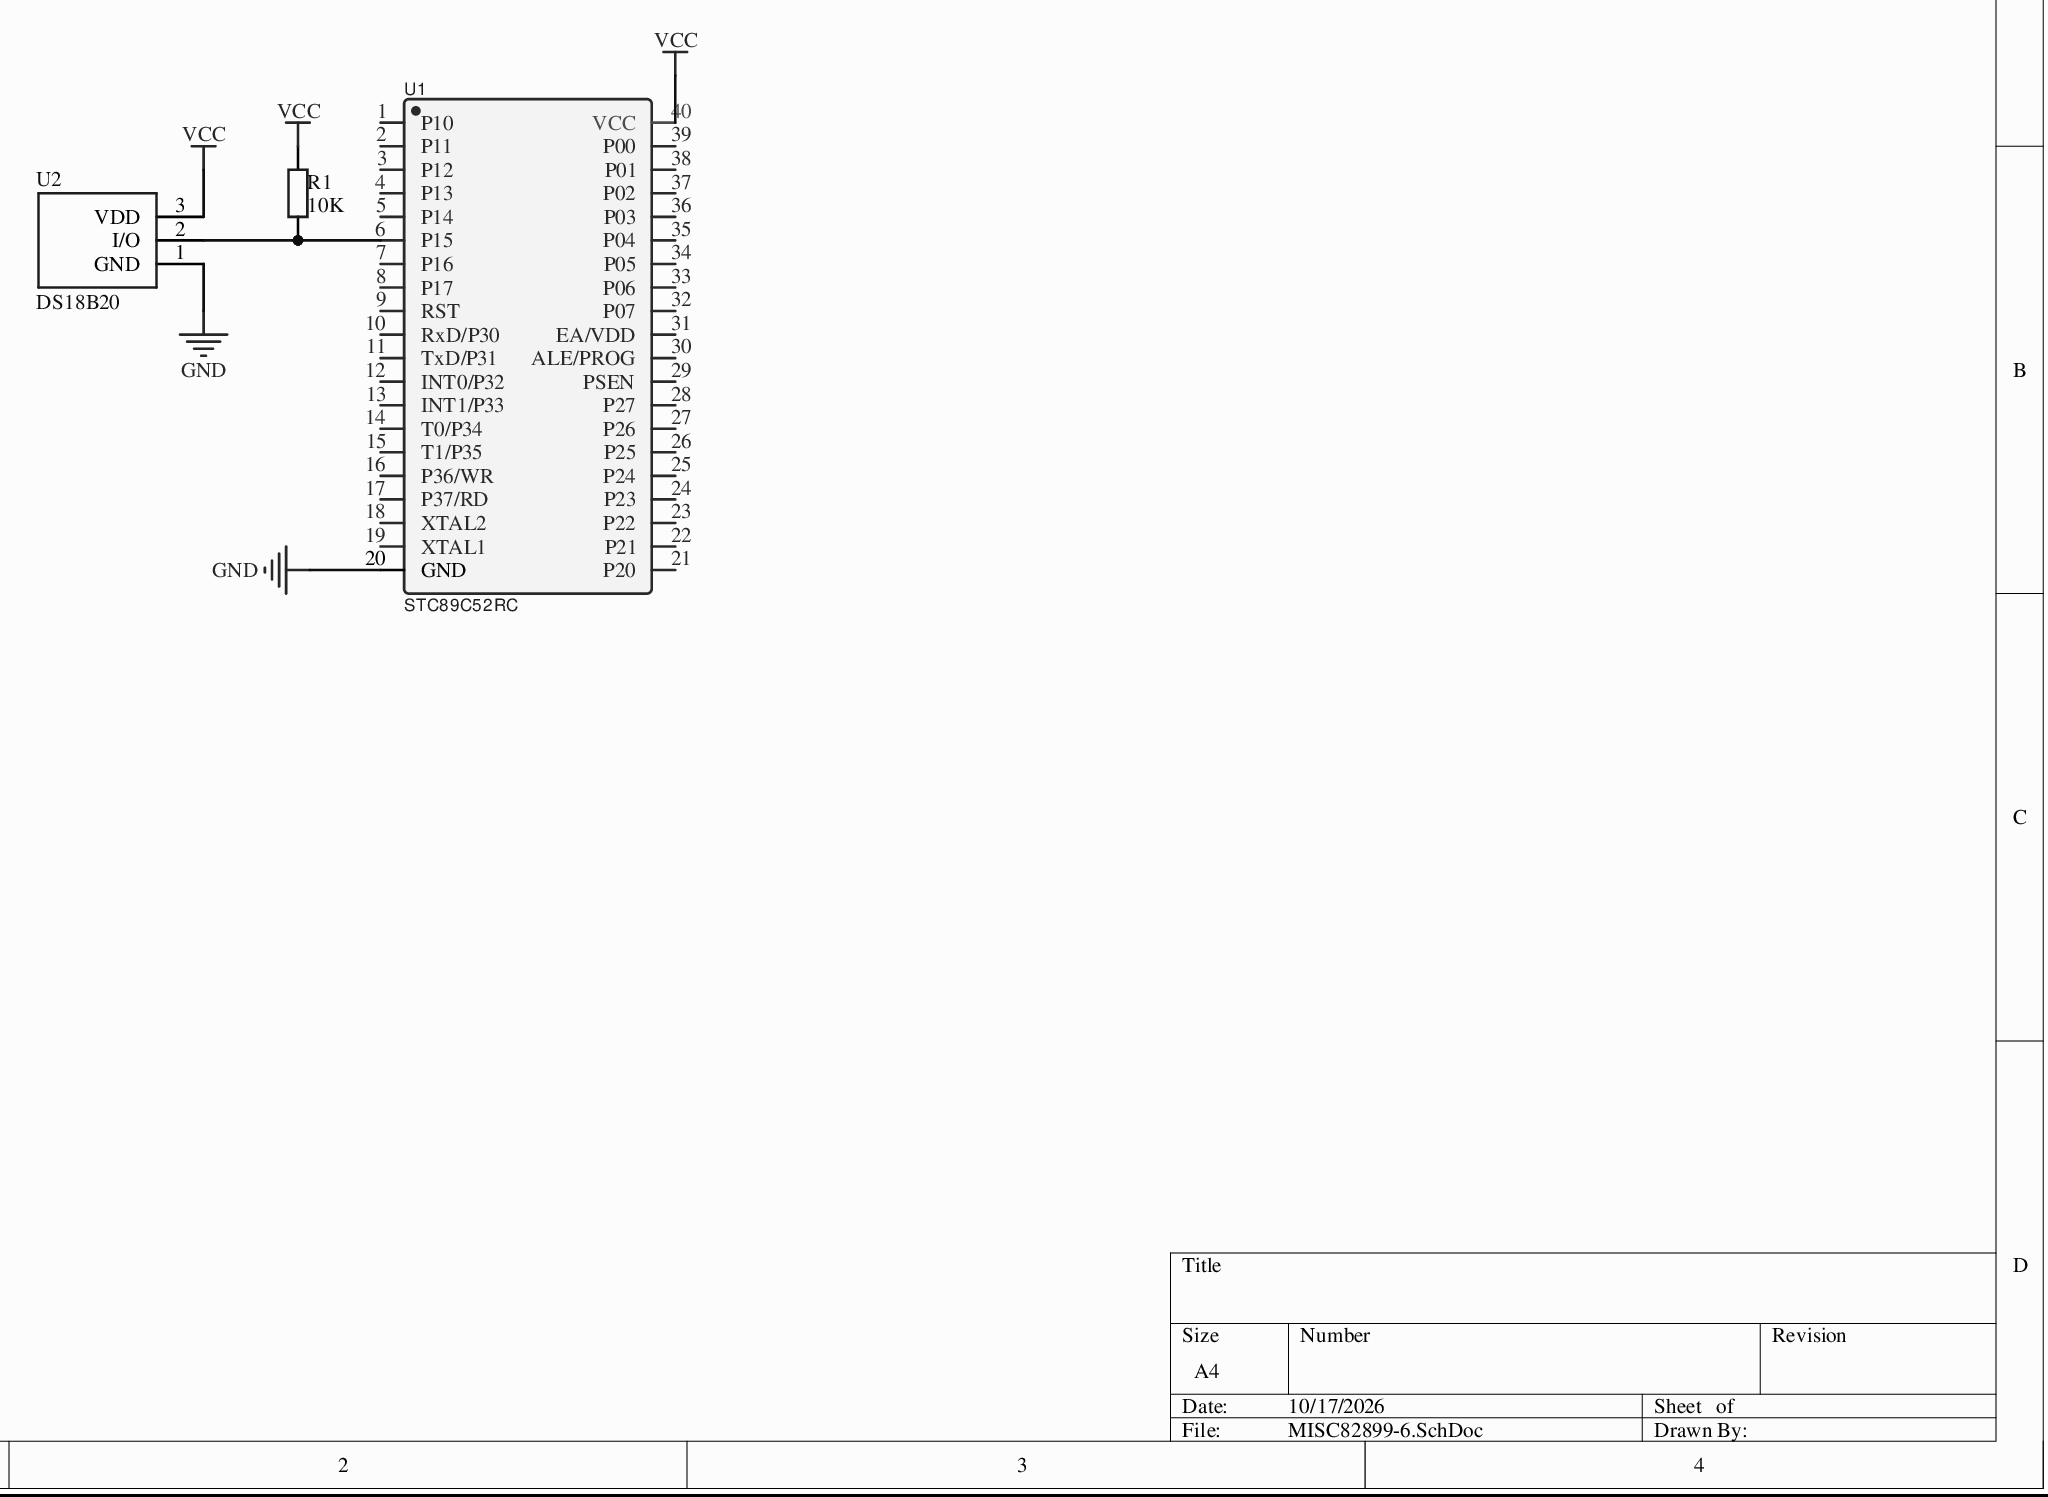
[diagram p0: MISC82899-6.SchDoc]
# Altium project MISC82899-2.PrjPcb
1 sheet, 3 parts. Net scope: global (net labels, ports and power ports of the same name join across sheets).
Board file: MISC82899.PcbDoc

## Sheet MISC82899-6.SchDoc
size A4

### Parts
R1  10K  [AXIAL-0.4]
U1  STC89C52RC  [STC89C52RC]
U2  DS18B20  [DS18B20]

### Nets
GND: U1.20(GND) U2.1(GND)
VCC: R1.2 U1.40(VCC) U2.3(VDD)
NetR1_1: R1.1 U1.6(P15) U2.2(I/O)

Not connected (* = marked no-connect by the designer): U1 1(P10) 2(P11) 3(P12) 4(P13) 5(P14) 7(P16) 8(P17) 9(RST) 10(RxD/P30) 11(TxD/P31) 12(INT0/P32) 13(INT1/P33) 14(T0/P34) 15(T1/P35) 16(P36/WR) 17(P37/RD) 18(XTAL2) 19(XTAL1) 21(P20) 22(P21) 23(P22) 24(P23) 25(P24) 26(P25) 27(P26) 28(P27) 29(PSEN) 30(ALE/PROG) 31(EA/VDD) 32(P07) 33(P06) 34(P05) 35(P04) 36(P03) 37(P02) 38(P01) 39(P00)

### Library data of the parts
R1 = Res2: Resistor; Value: 1K; Published: 8-Jun-2000; LatestRevisionDate: 17-Jul-2002; LatestRevisionNote: Re-released for DXP Platform.; PackageReference: AXIAL-0.4; PackageDescription: Axial Device, Thru-Hole; 2 Leads; 0.4 in Pin Spacing; Publisher: Altium Limited